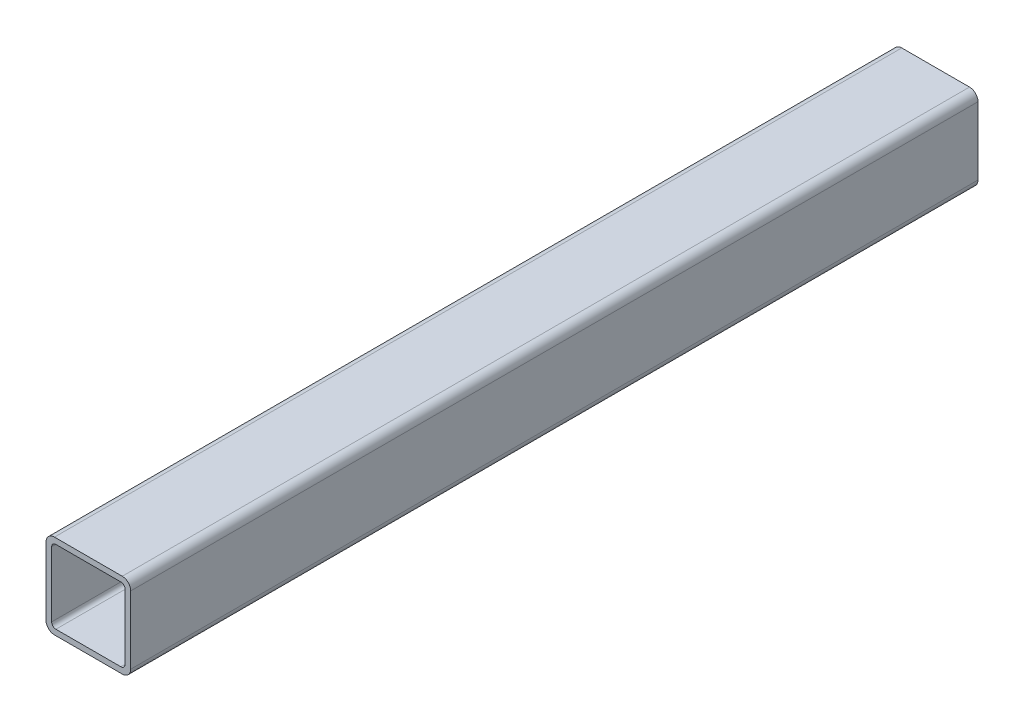
SolidWorks part; units mm, degrees
material "Q235"
ref_plane "Front Plane" through (0, 0, 0) normal (0, 0, 1) x (1, 0, 0)
ref_plane "Top Plane" through (0, 0, 0) normal (0, 1, 0) x (1, 0, 0)
ref_plane "Right Plane" through (0, 0, 0) normal (1, 0, 0) x (0, 0, -1)
sketch "Sketch1" plane through (0, 0, 0) normal (0, 0, 1) x (1, 0, 0)
  line L1 (-30, -30) -> (30, -30)
  line L2 (-30, -30) -> (-30, 30)
  line L3 (-30, 30) -> (30, 30)
  line L4 (30, -30) -> (30, 30)
  line L5 (-30, -30) -> (30, 30) construction
  line L6 (-30, 30) -> (30, -30) construction
  line L7 (-26, -26) -> (26, -26)
  line L8 (-26, -26) -> (-26, 26)
  line L9 (-26, 26) -> (26, 26)
  line L10 (26, -26) -> (26, 26)
  line L11 (-26, -26) -> (26, 26) construction
  line L12 (-26, 26) -> (26, -26) construction
  point P0 (0, 0)
  point P5 (0, 0)
  dimension "D1" = 4
  dimension "D2" = 60
  dimension "D3" = 60
extrude "Boss-Extrude1" add sketch "Sketch1" along normal blind 600
fillet "Fillet1" radius 6 4 edges at (30, -30, 300) (-30, -30, 300) (30, 30, 300) (-30, 30, 300)
fillet "Fillet2" radius 3 4 edges at (26, -26, 300) (-26, -26, 300) (26, 26, 300) (-26, 26, 300)
